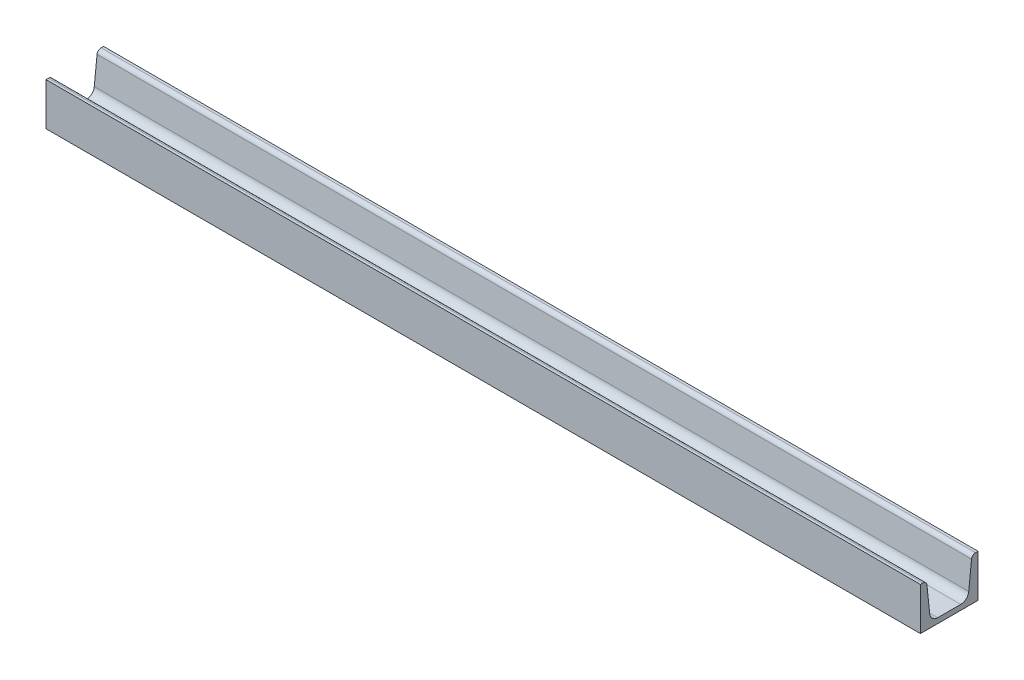
SolidWorks part; units mm, degrees
material "AISI 304"
ref_plane "Front Plane" through (0, 0, 0) normal (0, 0, 1) x (1, 0, 0)
ref_plane "Top Plane" through (0, 0, 0) normal (0, 1, 0) x (1, 0, 0)
ref_plane "Right Plane" through (0, 0, 0) normal (1, 0, 0) x (0, 0, -1)
other "Configuration Table"
sketch "草图1" plane through (0, 0, 0) normal (0, 0, 1) x (1, 0, 0)
  line L0 (-380, 0) -> (380, 0)
  point P4 (0, 0)
  dimension "D1" = 760
other "GB/T 707-1988 hot-rolled channel 05(1)"
ref_plane "Plane1" through (-380, 0, 0) normal (1, 0, 0) x (0, 1, 0)
sketch "Sketch1" plane through (-380, 0, 0) normal (1, 0, 0) x (0, 1, 0)
  line L0 (37, 50) -> (0, 50)
  line L1 (37, 0) -> (0, 0)
  line L2 (0, 50) -> (0, 0)
  line L3 (-9.5694, 25) -> (49.7414, 25) construction
  line L4 (4.5, 34.9892) -> (4.5, 15.0108)
  line L5 (37, 0) -> (37, 2.1406)
  line L6 (37, 50) -> (37, 47.8594)
  line L7 (10.7683, 8.0491) -> (33.8658, 5.6215)
  line L17 (10.7683, 41.9509) -> (33.8658, 44.3785)
  arc A0 (33.8658, 44.3785) -> (37, 47.8594) centre (33.5, 47.8594) ccw
  arc A1 (33.8658, 5.6215) -> (37, 2.1406) centre (33.5, 2.1406) cw
  arc A2 (4.5, 15.0108) -> (10.7683, 8.0491) centre (11.5, 15.0108) ccw
  arc A10 (4.5, 34.9892) -> (10.7683, 41.9509) centre (11.5, 34.9892) cw
  point P6 (0, 0)
  point P8 (0, 25)
  point P9 (4.5, 25.8841)
  point P10 (18.5, 50)
  point P13 (37, 44.7079)
  point P14 (20.75, 43)
  point P19 (4.5, 25)
equation "\"RI@Sketch1\" = \"D1@Sketch1\""
equation "\"D3@Sketch1\" =  ( \"BF@Sketch1\" - \"D6@Sketch1\" )  / 2"
